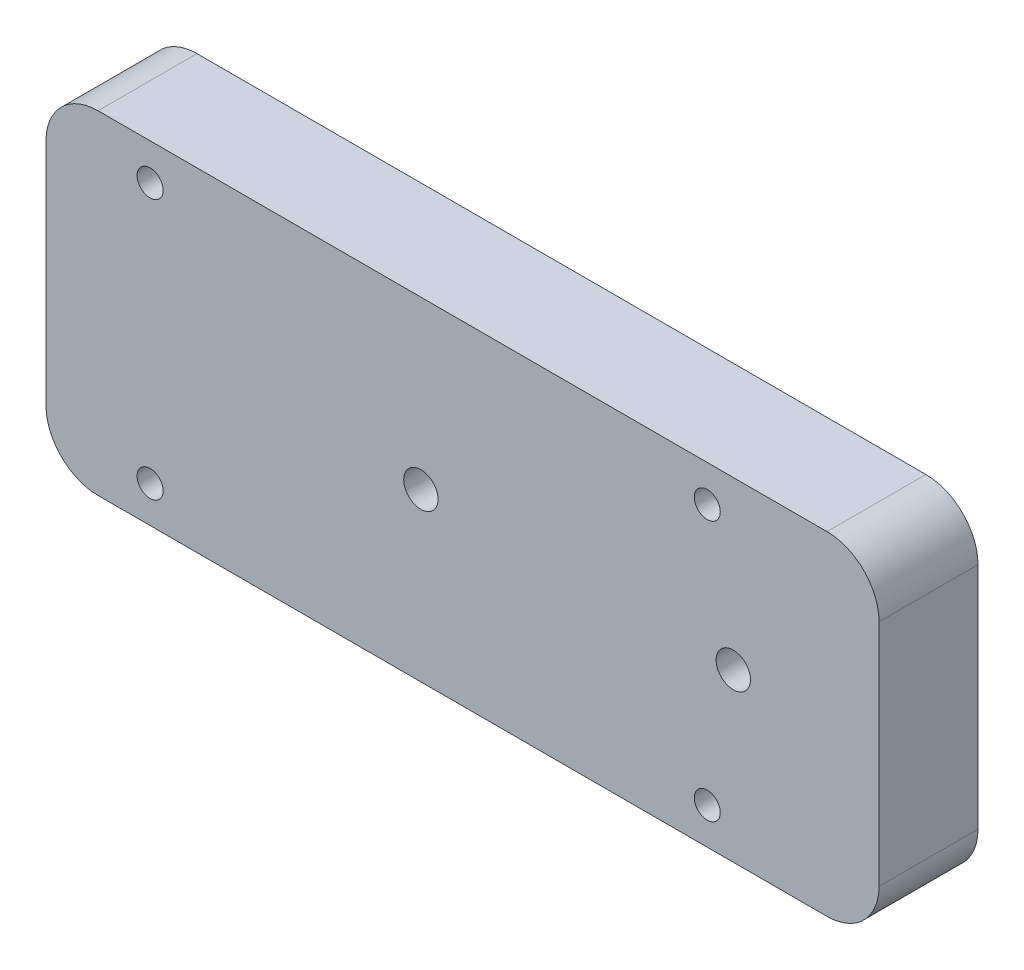
SolidWorks part; units mm, degrees
material "6061 GB/T6892-2006"
ref_plane "前视基准面" through (0, 0, 0) normal (0, 0, 1) x (1, 0, 0)
ref_plane "上视基准面" through (0, 0, 0) normal (0, 1, 0) x (1, 0, 0)
ref_plane "右视基准面" through (0, 0, 0) normal (1, 0, 0) x (0, 0, -1)
sketch "草图1" plane through (0, 0, 0) normal (0, 0, 1) x (1, 0, 0)
  line L5 (-80, 32) -> (80, 32)
  line L6 (-80, 32) -> (-80, -32)
  line L7 (-80, -32) -> (80, -32)
  line L8 (80, 32) -> (80, -32)
  line L9 (-80, 32) -> (80, -32) construction
  line L10 (-80, -32) -> (80, 32) construction
  point P0 (0, 0)
  dimension "D1" = 64
  dimension "D2" = 160
extrude "凸台-拉伸1" add sketch "草图1" along normal blind 19
fillet "圆角1" radius 10 4 edges at (80, 32, 9.5) (80, -32, 9.5) (-80, 32, 9.5) (-80, -32, 9.5)
hole_wizard "M6 螺纹孔1" positions "草图3" profile "草图4" tap size "M6" standard "GB" end condition through all
sketch "草图3" plane through (0, 0, 19) normal (0, 0, 1) x (1, 0, 0)
  line L0 (-80, 22) -> (-80, -22) construction
  line L3 (0, 0) -> (48.6927, 0) construction
  point P0 (-60, 25)
  point P2 (-60, -25)
  point P4 (47, 25)
  point P6 (47, -25)
  dimension "D1" = 20
  dimension "D2" = 50
  dimension "D3" = 20
  dimension "D4" = 107
sketch "草图4" plane through (-60, 25, 19) normal (1, 0, 0) x (0, -1, 0)
  line L0 (0, 0) -> (0, 19)
  line L1 (0, 19) -> (2.5, 19)
  line L2 (2.5, 19) -> (2.5, 0)
  line L5 (2.5, 0) -> (0, 0)
  line L11 (0, -6.35) -> (0, 107.95) construction
  dimension "通孔螺纹孔钻头直径" = 5
  dimension "通孔螺纹孔钻头深度" = 19
cosmetic thread "孔螺蚊线1"
cosmetic thread "孔螺蚊线2"
cosmetic thread "孔螺蚊线3"
cosmetic thread "孔螺蚊线4"
hole_wizard "打孔尺寸(%根据)内六角花形半沉头螺钉的类型2" positions "草图5" profile "草图6" countersink size "M6" standard "GB" end condition through all
sketch "草图5" plane through (0, 0, 0) normal (0, 0, -1) x (-1, 0, 0)
  line L0 (80, 22) -> (80, -22) construction
  point P0 (-52, 0)
  point P2 (8, 0)
  dimension "D1" = 72
  dimension "D2" = 60
sketch "草图6" plane through (52, 0, 0) normal (1, 0, 0) x (0, 1, 0)
  line L0 (0, 0) -> (0, 19)
  line L1 (0, 19) -> (3.3, 19)
  line L2 (3.3, 19) -> (3.3, 3.1)
  line L3 (3.3, 3.1) -> (6.4, 0)
  line L5 (6.4, 0) -> (0, 0)
  line L6 (-3.3, 3.1) -> (-6.4, 0) construction
  line L11 (0, -6.35) -> (0, 107.95) construction
  dimension "通孔孔直径" = 6.6
  dimension "通孔孔深度" = 19
  dimension "近端锥形沉头孔直径" = 12.8
  dimension "近端锥形沉头孔角度" = 90
